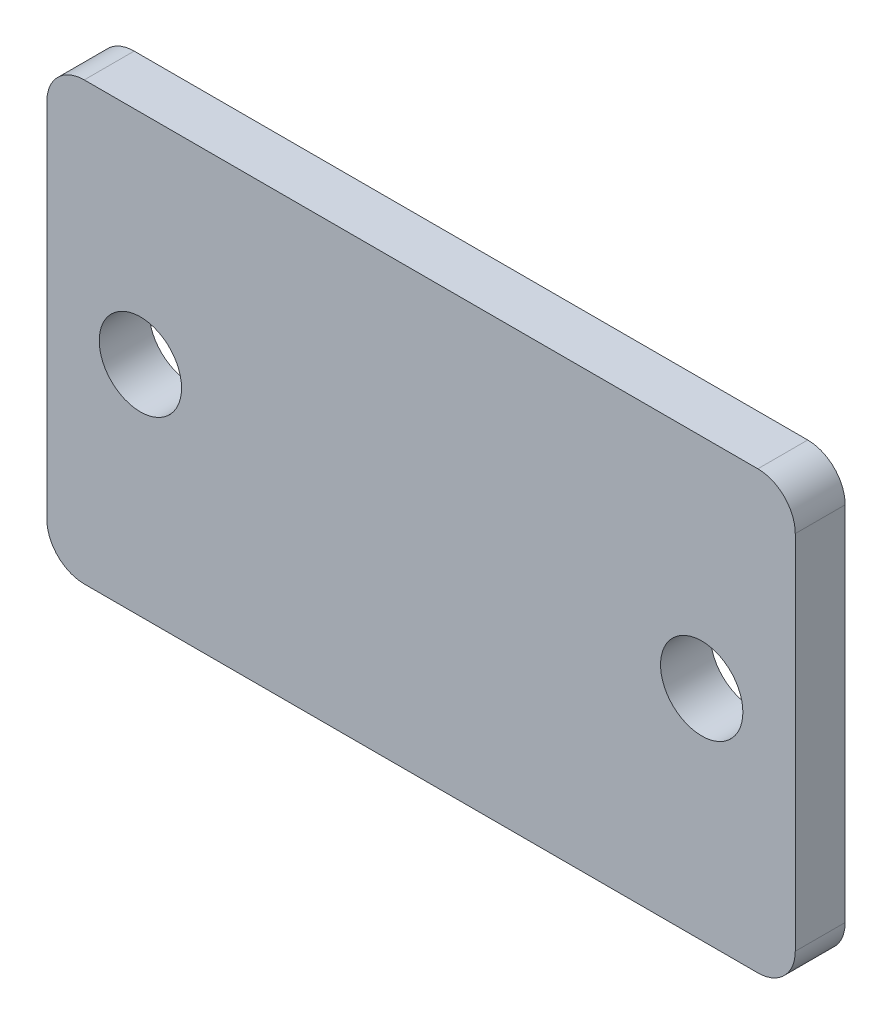
SolidWorks part; units mm, degrees
ref_plane "前视基准面" through (0, 0, 0) normal (0, 0, 1) x (1, 0, 0)
ref_plane "上视基准面" through (0, 0, 0) normal (0, 1, 0) x (1, 0, 0)
ref_plane "右视基准面" through (0, 0, 0) normal (1, 0, 0) x (0, 0, -1)
sketch "草图1" plane through (0, 0, 0) normal (0, 0, 1) x (1, 0, 0)
  line L0 (-22.5, 0) -> (0, 0) construction
  line L1 (-30, 17.5) -> (30, 17.5)
  line L2 (-30, 17.5) -> (-30, -17.5)
  line L3 (-30, -17.5) -> (30, -17.5)
  line L4 (30, 17.5) -> (30, -17.5)
  line L5 (-30, 17.5) -> (30, -17.5) construction
  line L6 (-30, -17.5) -> (30, 17.5) construction
  line L7 (0, 0) -> (22.5, 0) construction
  circle A0 centre (-22.5, 0) radius 3.3
  circle A1 centre (22.5, 0) radius 3.3
  point P0 (0, 0)
  dimension "D4" = 6.6
  dimension "D1" = 35
  dimension "D2" = 60
  dimension "D3" = 45
extrude "凸台-拉伸1" add sketch "草图1" along normal blind 4
fillet "圆角1" radius 3 4 edges at (30, -17.5, 2) (30, 17.5, 2) (-30, -17.5, 2) (-30, 17.5, 2)
